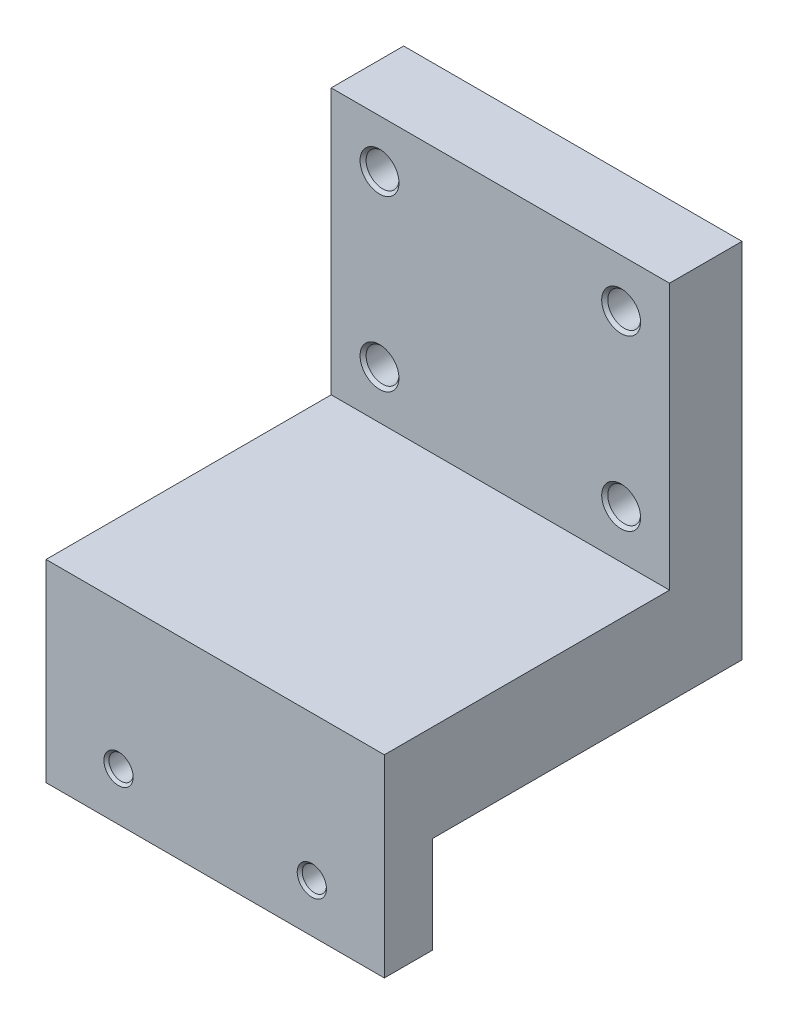
from build123d import *

# Parameters (mm, degrees)
EXTRUDE_1_DEPTH              = 10
EXTRUDE_1_DEPTH_BACK         = 64
SKETCH_1_W                   = 70
SKETCH_1_H                   = 20
SKETCH_2_W                   = 70
SKETCH_2_H                   = 10
EXTRUDE_2_DEPTH              = 20
SKETCH_3_W                   = 70
SKETCH_3_H                   = 15
EXTRUDE_3_DEPTH              = 55
HOLE_WIZARD_M8_1_D           = 6.8
HOLE_WIZARD_M8_1_DEPTH       = 17.707073895
HOLE_WIZARD_M8_1_CSINK_D     = 8.05
HOLE_WIZARD_M8_1_CSINK_ANGLE = 90
HOLE_WIZARD_M8_1_TIP         = 2.042926105
HOLE_WIZARD_M6_1_D           = 5
HOLE_WIZARD_M6_1_DEPTH       = 13.497848452
HOLE_WIZARD_M6_1_CSINK_D     = 6.05
HOLE_WIZARD_M6_1_CSINK_ANGLE = 90
HOLE_WIZARD_M6_1_TIP         = 1.502151548


with BuildPart() as part:
    # 草图1 → 凸台-拉伸1 (new, two sides: drawn at the far end of the back side and taken through both)
    with BuildSketch(Plane.XY.offset(-EXTRUDE_1_DEPTH_BACK)):
        with Locations((0, 45)):
            Rectangle(SKETCH_1_W, SKETCH_1_H)
    extrude(amount=EXTRUDE_1_DEPTH + EXTRUDE_1_DEPTH_BACK)

    # 草图2 → 凸台-拉伸2 (add)
    with BuildSketch(Plane.XZ.offset(-35)):
        with Locations((0, 5)):
            Rectangle(SKETCH_2_W, SKETCH_2_H)
    extrude(amount=EXTRUDE_2_DEPTH)

    # 草图3 → 凸台-拉伸3 (add)
    with BuildSketch(Plane(origin=(0, 55, 0), x_dir=(1, 0, 0), z_dir=(0, 1, 0))):
        with Locations((0, 56.5)):
            Rectangle(SKETCH_3_W, SKETCH_3_H)
    extrude(amount=EXTRUDE_3_DEPTH)

    # M8 螺纹孔1
    with Locations(Plane.XY.offset(-49)):
        with Locations((25, 100), (25, 65), (-25, 65), (-25, 100)):
            CounterSinkHole(HOLE_WIZARD_M8_1_D / 2, HOLE_WIZARD_M8_1_CSINK_D / 2, depth=HOLE_WIZARD_M8_1_DEPTH, counter_sink_angle=HOLE_WIZARD_M8_1_CSINK_ANGLE)
            with Locations((0, 0, -(HOLE_WIZARD_M8_1_DEPTH + HOLE_WIZARD_M8_1_TIP / 2))):  # 118° drill point
                Cone(0, HOLE_WIZARD_M8_1_D / 2, HOLE_WIZARD_M8_1_TIP, mode=Mode.SUBTRACT)

    # M6 螺纹孔1
    with Locations(Plane.XY.offset(10)):
        with Locations((20, 25), (-20, 25)):
            CounterSinkHole(HOLE_WIZARD_M6_1_D / 2, HOLE_WIZARD_M6_1_CSINK_D / 2, depth=HOLE_WIZARD_M6_1_DEPTH, counter_sink_angle=HOLE_WIZARD_M6_1_CSINK_ANGLE)
            with Locations((0, 0, -(HOLE_WIZARD_M6_1_DEPTH + HOLE_WIZARD_M6_1_TIP / 2))):  # 118° drill point
                Cone(0, HOLE_WIZARD_M6_1_D / 2, HOLE_WIZARD_M6_1_TIP, mode=Mode.SUBTRACT)


solid = part.part
